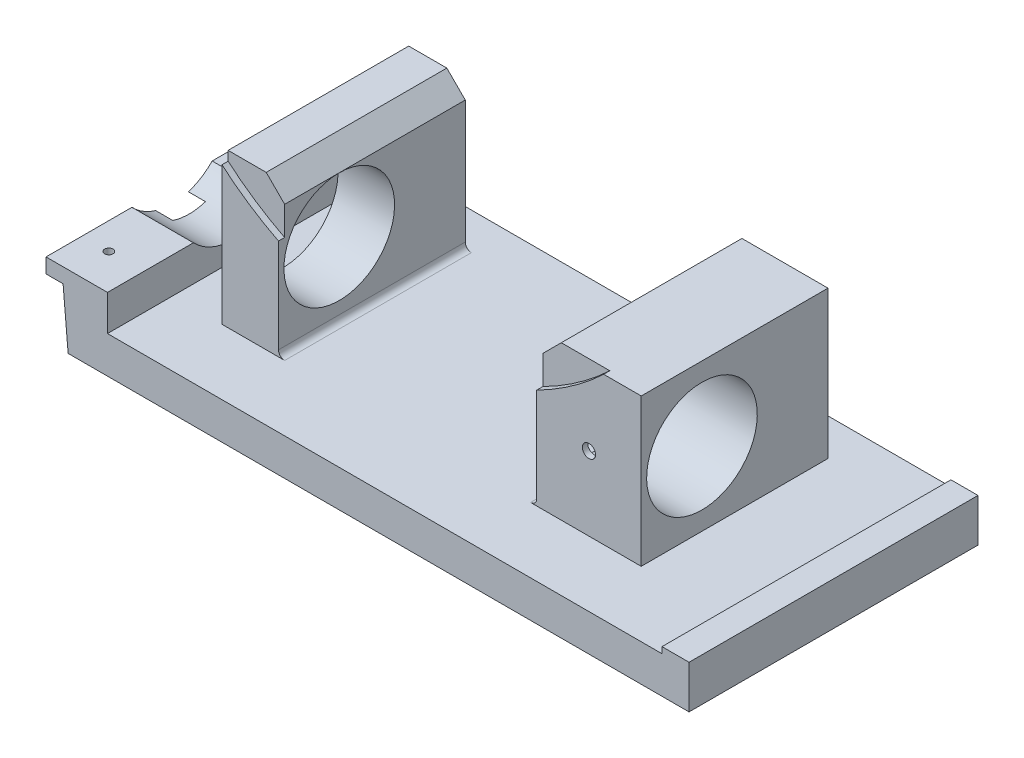
SolidWorks part; units mm, degrees
ref_plane "Front Plane" through (0, 0, 0) normal (0, 0, 1) x (1, 0, 0)
ref_plane "Top Plane" through (0, 0, 0) normal (0, 1, 0) x (1, 0, 0)
ref_plane "Right Plane" through (0, 0, 0) normal (1, 0, 0) x (0, 0, -1)
other "Configuration Table"
sketch "Sketch1" plane through (0, 0, 0) normal (0, 0, 1) x (1, 0, 0)
  line L0 (0, 0) -> (0, 318.5) construction
  line L1 (-227.112, 47) -> (-223, 0)
  line L2 (-223, 0) -> (282, 0)
  line L3 (282, 0) -> (282, 35)
  line L4 (-105, 30) -> (105, 30)
  line L5 (-105, 30) -> (-105, 148.2796)
  line L6 (105, 30) -> (105, 148.2796)
  line L7 (-151, 150) -> (-151, 30)
  line L8 (-191, 59) -> (-191, 30)
  line L9 (-151, 30) -> (-191, 30)
  line L10 (190, 150) -> (190, 30)
  line L11 (260, 35) -> (260, 30)
  line L12 (190, 30) -> (260, 30)
  line L13 (260, 35) -> (282, 35)
  line L15 (-151, 150) -> (-107.7393, 150)
  line L16 (107.7393, 150) -> (190, 150)
  line L17 (-179.2547, 318.5) -> (265.7439, 318.5) construction
  line L18 (-227.112, 47) -> (-241, 47)
  line L19 (-241, 47) -> (-241, 59)
  line L20 (-241, 59) -> (-191, 59)
  arc A0 (-107.7393, 150) -> (-105, 148.2796) centre (0, 318.5) ccw
  arc A1 (105, 148.2796) -> (107.7393, 150) centre (0, 318.5) ccw
  dimension "D14" = 200
  dimension "D1" = 223
  dimension "D2" = 70
  dimension "D3" = 95
  dimension "D4" = 30
  dimension "D5" = 105
  dimension "D6" = 105
  dimension "D7" = 46
  dimension "D8" = 40
  dimension "D9" = 85
  dimension "D10" = 22
  dimension "D11" = 35
  dimension "D12" = 47
  dimension "D13" = 318.5
  dimension "D15" = 150
  dimension "D16" = 150
  dimension "D17" = 50
  dimension "D18" = 12
extrude "Boss-Extrude1" add sketch "Sketch1" against normal blind 205
fillet "Fillet1" radius 5 2 edges at (105, 30, -102.5) (-105, 30, -102.5)
sketch "Sketch2" plane through (282, 0, 0) normal (1, 0, 0) x (0, 0, -1)
  line L0 (205, 0) -> (205, 35) construction
  line L1 (205, 0) -> (0, 0) construction
  circle A0 centre (102.5, 90) radius 45
  dimension "D2" = 90
  dimension "D1" = 102.5
  dimension "D3" = 90
extrude "Cut-Extrude1" cut sketch "Sketch2" against normal through all
ref_plane "Plane1" through (147.5, 0, 0) normal (1, 0, 0) x (0, 0, -1)
sketch "Sketch3" plane through (147.5, 0, 0) normal (1, 0, 0) x (0, 0, -1)
  line L0 (102.5, 90) -> (-39.0779, 90) construction
  line L9 (0, 95.9) -> (0, 90)
  line L10 (90, 95) -> (0, 95.9)
  line L11 (90, 90) -> (90, 95)
  line L12 (0, 90) -> (90, 90)
  line L13 (0, 95.9) -> (0, 90)
  line L14 (90, 95) -> (0, 95.9)
  line L15 (90, 90) -> (90, 95)
  line L16 (0, 90) -> (90, 90)
  dimension "D1" = 0
revolve "Cut-Revolve1" cut sketch "Sketch3" angle 360 about L0
sketch "Sketch4" plane through (0, 0, -205) normal (0, 0, -1) x (-1, 0, 0)
  line L0 (-120, 150) -> (-105, 135)
  line L1 (-190, 150) -> (-107.7393, 150) construction
  line L2 (-105, 148.2796) -> (-105, 35) construction
  line L3 (-105, 135) -> (-105, 150)
  line L4 (-105, 150) -> (-120, 150)
  line L5 (105, 150) -> (120, 150)
  line L6 (107.7393, 150) -> (151, 150) construction
  line L7 (120, 150) -> (105, 135)
  line L8 (105, 35) -> (105, 148.2796) construction
  line L9 (105, 135) -> (105, 150)
  dimension "D1" = 15
  dimension "D2" = 15
  dimension "D3" = 15
  dimension "D4" = 15
extrude "Cut-Extrude2" cut sketch "Sketch4" against normal through all
sketch "Sketch5" plane through (0, 0, -53.1) normal (0, 0, -1) x (-1, 0, 0)
  circle A0 centre (0, 318.5) radius 232
  circle A1 centre (0, 318.5) radius 227 construction
  dimension "D1" = 5
extrude "Cut-Extrude3" cut sketch "Sketch5" against normal through all and the other way blind 5
sketch "Sketch6" plane through (0, 0, -205) normal (0, 0, -1) x (-1, 0, 0)
  line L0 (-282, 0) -> (223, 0)
  line L1 (223, 0) -> (227.112, 47)
  line L2 (227.112, 47) -> (241, 47)
  line L3 (241, 47) -> (241, 59)
  line L4 (241, 59) -> (191, 59)
  line L5 (191, 59) -> (191, 30)
  line L6 (191, 30) -> (-260, 30)
  line L7 (-260, 30) -> (-260, 35)
  line L8 (-260, 35) -> (-282, 35)
  line L9 (-282, 35) -> (-282, 0)
extrude "Boss-Extrude2" add sketch "Sketch6" along normal blind 30
sketch "Sketch7" plane through (0, 0, 0) normal (0, 0, 1) x (1, 0, 0)
  line L0 (-151, 30) -> (-151, 146.1833)
  line L1 (-151, 150) -> (-151, 142.3665) construction
  line L2 (-151, 146.1833) -> (-120, 150)
  line L3 (-120, 150) -> (-105, 135)
  line L4 (-105, 135) -> (-105, 35)
  line L5 (-105, 35) -> (-100, 30)
  line L6 (-100, 30) -> (-151, 30)
  line L7 (190, 150) -> (190, 30)
  line L8 (190, 30) -> (100, 30)
  line L9 (100, 30) -> (105, 35)
  line L10 (105, 35) -> (105, 135)
  line L11 (105, 135) -> (120, 150)
  line L12 (120, 150) -> (190, 150)
extrude "Cut-Extrude4" cut sketch "Sketch7" against normal blind 53.1
hole_wizard "M8 Tapped Hole1" positions "Sketch8" profile "Sketch9" tap size "M8" standard "GB"
sketch "Sketch8" plane through (0, 59, 0) normal (0, 1, 0) x (1, 0, 0)
  point P0 (271, 29.3637)
  point P3 (271, 219.9532)
  point P5 (-219.3032, 219.9981)
  point P8 (-219.3032, 29.3637)
sketch "Sketch9" plane through (271, 59, -29.3637) normal (1, 0, 0) x (0, 0, 1)
  line L0 (0, 0) -> (0, 22.25)
  line L1 (0, 22.25) -> (3.4, 20.2071)
  line L2 (3.4, 20.2071) -> (3.4, 0)
  line L5 (3.4, 0) -> (0, 0)
  line L10 (0, 22.25) -> (-3.4, 20.2071) construction
  line L11 (0, -6.35) -> (0, 107.95) construction
  dimension "螺纹孔钻头直径" = 6.8
  dimension "螺纹孔钻头深度" = 22.25
  dimension "导头角度" = 118
cosmetic thread "Cosmetic Thread1" parameters "D1"=16, "D2"=8
cosmetic thread "Cosmetic Thread2" parameters "D1"=16, "D2"=8
